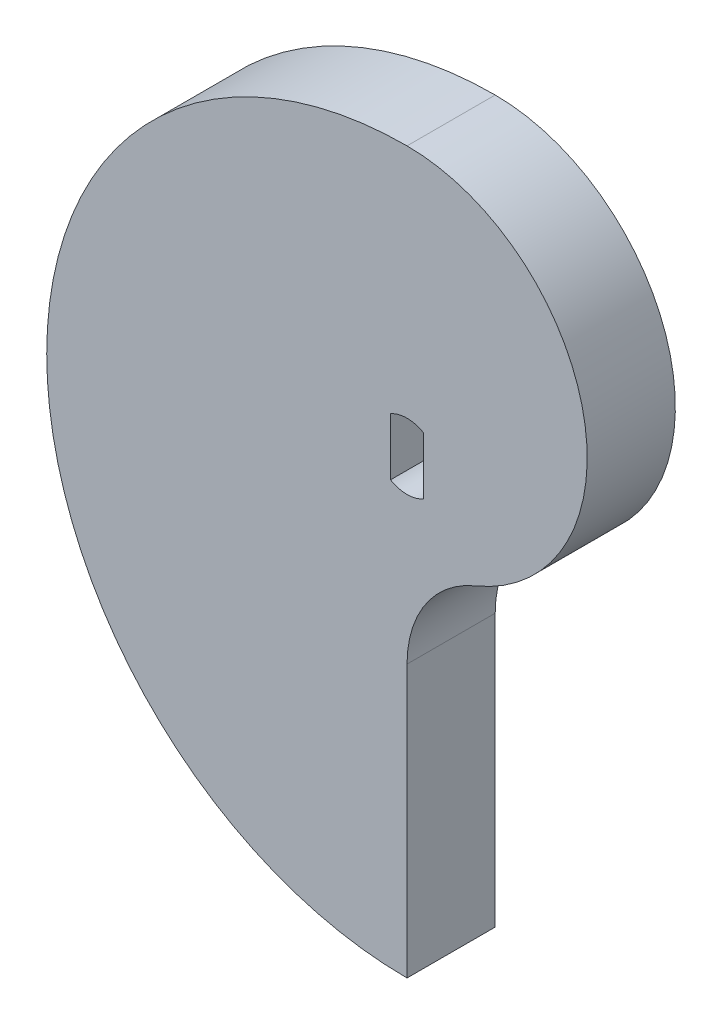
SolidWorks part; units mm, degrees
ref_plane "Front Plane" through (0, 0, 0) normal (0, 0, 1) x (1, 0, 0)
ref_plane "Top Plane" through (0, 0, 0) normal (0, 1, 0) x (1, 0, 0)
ref_plane "Right Plane" through (0, 0, 0) normal (1, 0, 0) x (0, 0, -1)
sketch "Sketch4" plane through (0, 0, 0) normal (0, 0, 1) x (1, 0, 0)
  line L2 (0, -20.5) -> (0, -4.15)
  arc A2 (0, 12.2) -> (0, -20.5) centre (0, -4.15) ccw
  circle A3 centre (0, 0) radius 2.5
  arc A5 (0, -4.15) -> (0, 12.2) centre (0, 4.025) ccw
extrude "Boss-Extrude3" add sketch "Sketch4" along normal blind 4
fillet "Fillet2" radius 5 1 edges at (0, -4.15, 2)
sketch "Sketch7" plane through (0, 0, 4) normal (0, 0, 1) x (1, 0, 0)
  circle A0 centre (0, 0) radius 1.5
  circle A2 centre (0, 0) radius 3.9862
extrude "Boss-Extrude4" add sketch "Sketch7" against normal blind 4
sketch "Sketch8" plane through (0, 0, 4) normal (0, 0, 1) x (1, 0, 0)
  line L0 (0, 0) -> (0, 1.5) construction
  line L1 (0, 1.118) -> (-1, 1.118) construction
  line L2 (0, 0) -> (-1, 1.118)
  line L3 (0, 0) -> (1.118, 1)
  line L4 (1.118, 1) -> (0.9961, 2.0287)
  line L5 (0.9961, 2.0287) -> (-1.0752, 1.9908)
  line L6 (-1.0752, 1.9908) -> (-1, 1.118)
  circle A0 centre (0, 0) radius 1.5 construction
extrude "Boss-Extrude5" add sketch "Sketch8" against normal blind 4
sketch "Sketch9" plane through (0, 0, 4) normal (0, 0, 1) x (1, 0, 0)
  circle A0 centre (0, 0) radius 1.5
extrude "Cut-Extrude1" cut sketch "Sketch9" against normal through all
sketch "Sketch10" plane through (0, 0, 4) normal (0, 0, 1) x (1, 0, 0)
  line L0 (-1.5, 0) -> (1.5, 0) construction
  line L1 (0, 1.5) -> (0, -1.5) construction
  line L2 (0, 1.299) -> (-0.75, 1.299)
  line L3 (0, 1.299) -> (0.75, 1.299)
  line L4 (-0.75, 1.299) -> (-0.75, -1.299)
  line L5 (0.75, 1.299) -> (0.75, -1.299)
  circle A2 centre (0, 0) radius 1.5
  circle M4 centre (0, 0) radius 1.5
extrude "Boss-Extrude6" add sketch "Sketch10" against normal through all contours L5 M4 | L4 M4
